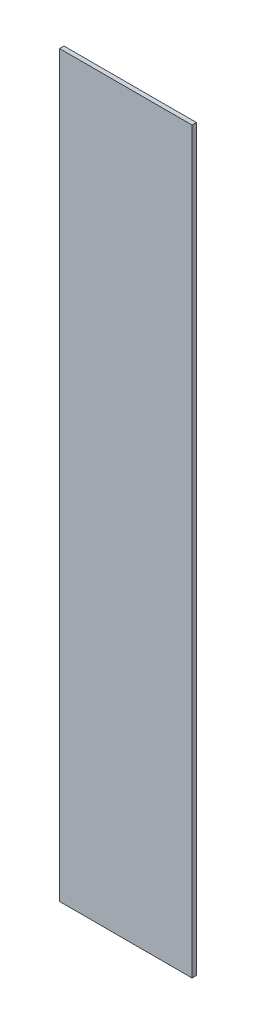
from build123d import *

# Parameters (mm, degrees)
SKETCH_1_W      = 151
SKETCH_1_H      = 842
EXTRUDE_1_DEPTH = 5


with BuildPart() as part:
    # 草图1 → 凸台-拉伸1 (new body)
    with BuildSketch(Plane.XY):
        Rectangle(SKETCH_1_W, SKETCH_1_H)
    extrude(amount=EXTRUDE_1_DEPTH)


solid = part.part
